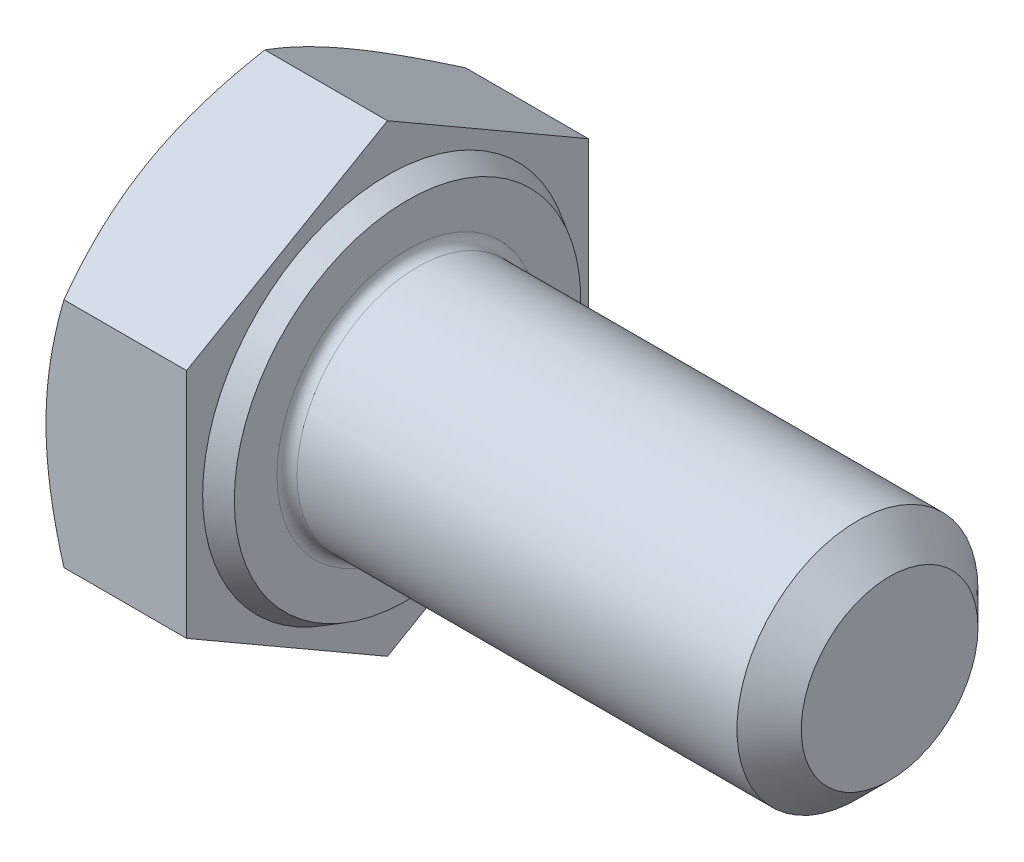
from build123d import *

# Parameters (mm, degrees)
BASE_EXTRUDE_DEPTH = 4
CHAMFER_2_SIZE     = 0.8


with BuildPart() as part:
    # Sketch1 → Base-extrude (new body)
    with BuildSketch(Plane(origin=(0, 0, 0), x_dir=(0, 0, -1), z_dir=(1, 0, 0))):
        Polygon((5, 2.886751346), (5, -2.886751346), (0, -5.773502692), (-5, -2.886751346), (-5, 2.886751346), (0, 5.773502692), align=None)
    extrude(amount=BASE_EXTRUDE_DEPTH)

    # Sketch2 → Boss-Revolve1 (revolve)
    with BuildSketch(Plane.XY, mode=Mode.PRIVATE) as boss_revolve1_sk:
        Polygon((0, 0), (16, 0), (16, 2.134), (16, 3), (4, 3), (0, 3), align=None)
    revolve(boss_revolve1_sk.sketch.rotate(Axis((0, 0, 0), (-1, 0, 0)), 90), axis=Axis((0, 0, 0), (-1, 0, 0)))

    # Sketch3 → Cut-Revolve1 (revolve, cut)
    with BuildSketch(Plane.XY):
        Polygon((0, 5), (3.333333333, 10.773502692), (3.333333333, 15.773502692), (-10, 15.773502692), (-10, 5), align=None)
    revolve(axis=Axis((0, 0, 0), (1, 0, 0)), mode=Mode.SUBTRACT)

    # Sketch5 → Cut-Revolve2 (revolve, cut)
    with BuildSketch(Plane.XY):
        Polygon((4, 5), (0.666666667, 10.773502692), (0.666666667, 15.773502692), (10.666666667, 15.773502692), (10.666666667, 5), align=None)
    revolve(axis=Axis((0, 0, 0), (1, 0, 0)), mode=Mode.SUBTRACT)

    # Sketch4 → Cut-Revolve3 (revolve, cut)
    with BuildSketch(Plane.XY, mode=Mode.PRIVATE) as cut_revolve3_sk:
        Polygon((4, 4.312264973), (3.5, 4.600940108), (3.5, 15.773502692), (4, 15.773502692), align=None)
    revolve(cut_revolve3_sk.sketch.rotate(Axis((0, 0, 0), (1, 0, 0)), 90), axis=Axis((0, 0, 0), (1, 0, 0)), mode=Mode.SUBTRACT)

    # Chamfer 2
    chamfer_2_edges = [part.edges().sort_by_distance(p)[0] for p in [
        (16, 0, 3),
    ]]
    chamfer(chamfer_2_edges, length=CHAMFER_2_SIZE)

    # Sketch9 → Revolve1 (revolve)
    with BuildSketch(Plane.XY, mode=Mode.PRIVATE) as revolve1_sk:
        with BuildLine():
            Line((4, 3.25), (4, 3))
            Line((4, 3), (4.25, 3))
            ThreePointArc((4.25, 3), (4.073223305, 3.073223305), (4, 3.25))
        make_face()
    revolve(revolve1_sk.sketch.rotate(Axis((0, 0, 0), (1, 0, 0)), 90), axis=Axis((0, 0, 0), (1, 0, 0)))


solid = part.part
